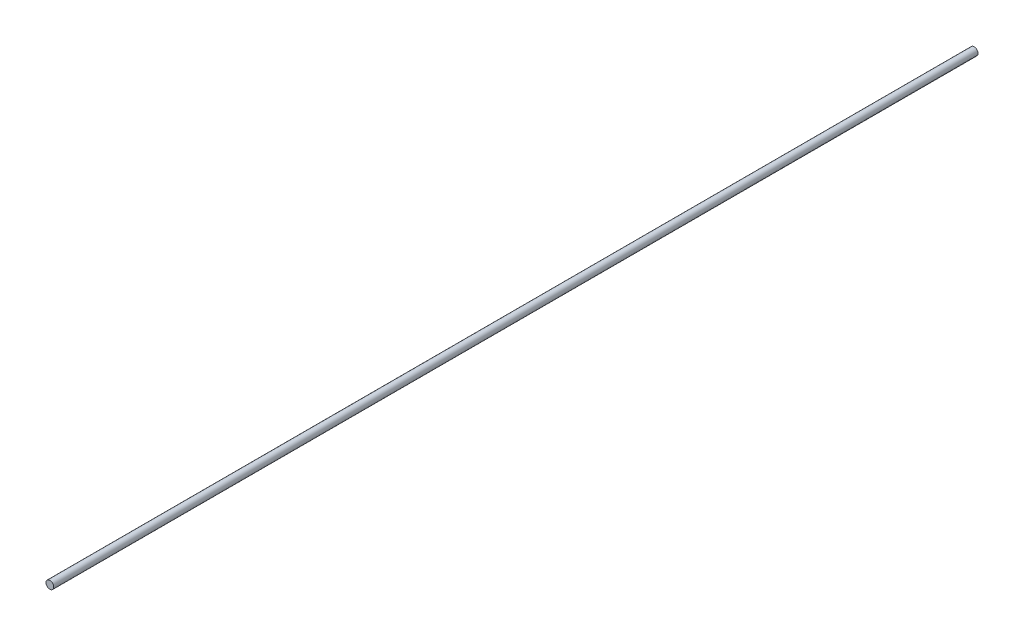
from build123d import *

# Parameters (mm, degrees)
SKETCH1_R           = 2
BOSS_EXTRUDE1_DEPTH = 479.4


with BuildPart() as part:
    # Sketch1 → Boss-Extrude1 (new body)
    with BuildSketch(Plane.XY):
        Circle(SKETCH1_R)
    extrude(amount=BOSS_EXTRUDE1_DEPTH)


solid = part.part
